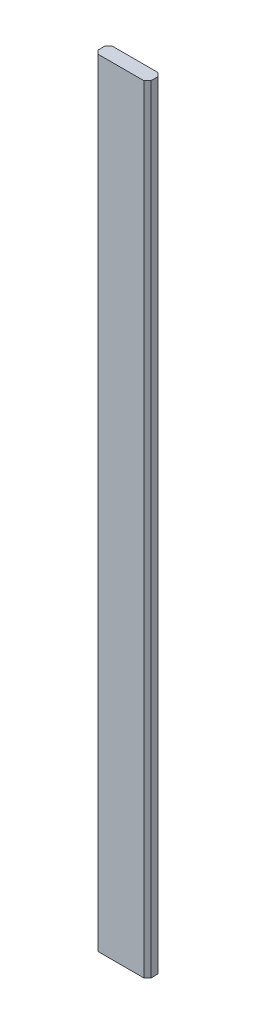
SolidWorks part; units mm, degrees
ref_plane "Front Plane" through (0, 0, 0) normal (0, 0, 1) x (1, 0, 0)
ref_plane "Top Plane" through (0, 0, 0) normal (0, 1, 0) x (1, 0, 0)
ref_plane "Right Plane" through (0, 0, 0) normal (1, 0, 0) x (0, 0, -1)
sketch "Sketch1" plane through (0, 0, 0) normal (0, 0, 1) x (1, 0, 0)
  line L1 (7.5, 110) -> (-7.5, 110)
  line L2 (7.5, 110) -> (7.5, -110)
  line L3 (7.5, -110) -> (-7.5, -110)
  line L4 (-7.5, 110) -> (-7.5, -110)
  line L5 (7.5, 110) -> (-7.5, -110) construction
  line L6 (7.5, -110) -> (-7.5, 110) construction
  point P0 (0, 0)
  dimension "D1" = 15
  dimension "D2" = 220
extrude "Boss-Extrude1" add sketch "Sketch1" along normal blind 4
chamfer "Chamfer1" distance 1 angle 45 4 edges at (-7.5, 0, 0) (7.5, 0, 0) (-7.5, 0, 4) (7.5, 0, 4)
